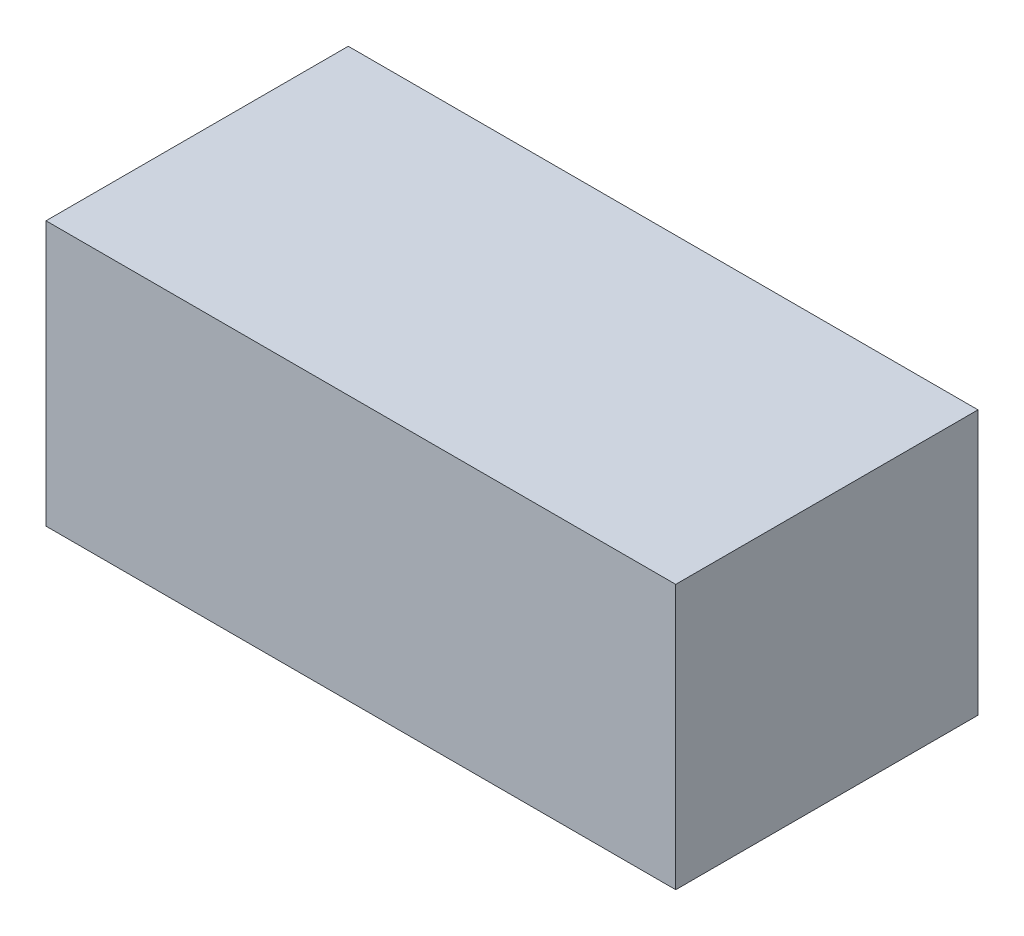
SolidWorks part; units mm, degrees
ref_plane "前视基准面" through (0, 0, 0) normal (0, 0, 1) x (1, 0, 0)
ref_plane "上视基准面" through (0, 0, 0) normal (0, 1, 0) x (1, 0, 0)
ref_plane "右视基准面" through (0, 0, 0) normal (1, 0, 0) x (0, 0, -1)
other "Configuration Table"
sketch "草图1" plane through (0, 0, 0) normal (0, 0, 1) x (1, 0, 0)
  line L0 (-12.5, -5.25) -> (12.5, -5.25)
  line L1 (12.5, -5.25) -> (12.5, 5.25)
  line L2 (12.5, 5.25) -> (-12.5, 5.25)
  line L3 (-12.5, 5.25) -> (-12.5, -5.25)
  point P0 (0, 0)
  dimension "D1" = 12.5
  dimension "D2" = 25
  dimension "D3" = 5.25
  dimension "D4" = 10.5
extrude "凸台-拉伸1" add sketch "草图1" against normal mid plane 12
